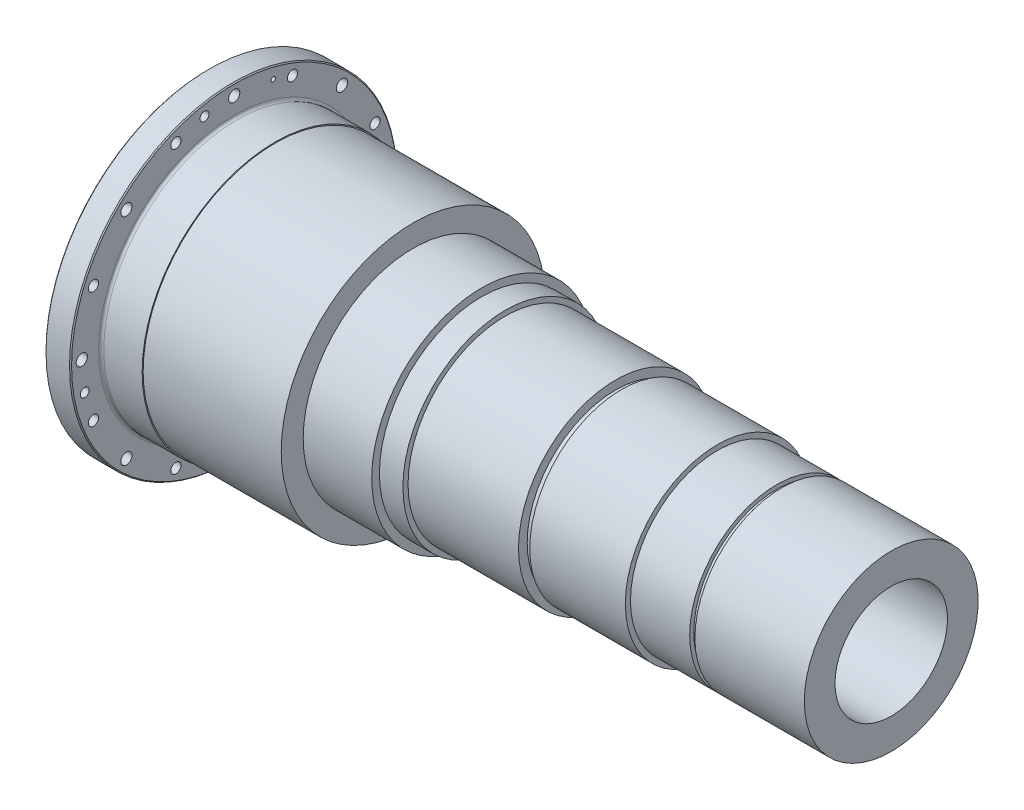
SolidWorks part; units mm, degrees
material "1.2311 (40CrMnMo7)"
ref_plane "Front Plane" through (0, 0, 0) normal (0, 0, 1) x (1, 0, 0)
ref_plane "Top Plane" through (0, 0, 0) normal (0, 1, 0) x (1, 0, 0)
ref_plane "Right Plane" through (0, 0, 0) normal (1, 0, 0) x (0, 0, -1)
sketch "Sketch1" plane through (0, 0, 0) normal (0, 0, 1) x (1, 0, 0)
  line L0 (0, 0) -> (1527.2972, 0) construction
  line L1 (0, 203) -> (0, 318)
  line L2 (2, 320) -> (48, 320)
  line L3 (50, 318) -> (50, 265)
  line L4 (55, 260) -> (130, 260)
  line L5 (130, 260) -> (130, 258)
  line L6 (130, 258) -> (400, 258)
  line L7 (400, 258) -> (400, 215)
  line L8 (400, 215) -> (534, 215)
  line L9 (534, 215) -> (534, 200)
  line L10 (534, 200) -> (580, 200)
  line L11 (580, 200) -> (580, 190)
  line L12 (580, 190) -> (796, 190)
  line L13 (796, 190) -> (796, 173)
  line L14 (796, 173) -> (808, 173)
  line L15 (808, 173) -> (808, 180)
  line L16 (808, 180) -> (995, 180)
  line L17 (995, 180) -> (995, 170)
  line L18 (995, 170) -> (1110.8, 170)
  line L19 (1110.8, 170) -> (1110.8, 162)
  line L21 (1335, 170) -> (1335, 110)
  line L22 (1335, 110) -> (874, 110)
  line L23 (874, 110) -> (864, 120)
  line L24 (864, 120) -> (413, 120)
  line L25 (413, 120) -> (413, 107.5)
  line L26 (413, 107.5) -> (353, 107.5)
  line L27 (353, 107.5) -> (353, 159)
  line L28 (353, 159) -> (340, 159)
  line L29 (340, 159) -> (340, 185)
  line L30 (340, 185) -> (283, 185)
  line L31 (283, 185) -> (283, 200)
  line L32 (278, 205) -> (175, 205)
  line L33 (170, 200) -> (170, 190)
  line L34 (170, 190) -> (110, 190)
  line L35 (110, 190) -> (110, 197)
  line L36 (107, 200) -> (3, 200)
  line L37 (1110.8, 162) -> (1121, 162)
  line L38 (1121, 162) -> (1121, 170)
  line L39 (1121, 170) -> (1335, 170)
  line L40 (3, 200) -> (0, 203)
  line L41 (0, 318) -> (2, 320)
  line L42 (48, 320) -> (50, 318)
  arc A0 (50, 265) -> (55, 260) centre (55, 265) ccw
  arc A1 (110, 197) -> (107, 200) centre (107, 197) ccw
  arc A2 (283, 200) -> (278, 205) centre (278, 200) ccw
  arc A3 (175, 205) -> (170, 200) centre (175, 200) ccw
  point P4 (0, 320)
  point P5 (50, 320)
  point P39 (0, 200)
  dimension "D38" = 5
  dimension "D39" = 3
  dimension "D43" = 5
  dimension "D1" = 320
  dimension "D2" = 1335
  dimension "D3" = 10.2
  dimension "D4" = 325
  dimension "D5" = 162
  dimension "D6" = 170
  dimension "D7" = 180
  dimension "D8" = 199
  dimension "D9" = 173
  dimension "D10" = 12
  dimension "D11" = 110
  dimension "D12" = 995
  dimension "D13" = 190
  dimension "D14" = 120
  dimension "D15" = 45
  dimension "D16" = 864
  dimension "D17" = 46
  dimension "D18" = 534
  dimension "D19" = 200
  dimension "D20" = 215
  dimension "D21" = 107.5
  dimension "D22" = 200
  dimension "D23" = 190
  dimension "D24" = 110
  dimension "D25" = 60
  dimension "D26" = 113
  dimension "D27" = 205
  dimension "D28" = 185
  dimension "D29" = 60
  dimension "D30" = 353
  dimension "D31" = 13
  dimension "D32" = 159
  dimension "D33" = 400
  dimension "D34" = 258
  dimension "D35" = 260
  dimension "D36" = 80
  dimension "D37" = 50
revolve "Revolve1" add sketch "Sketch1" angle 360 about L0
sketch "Sketch3" plane through (0, 0, 0) normal (-1, 0, 0) x (0, 0, 1)
  line L0 (0, 0) -> (114.0397, 275.3161) construction
  line L1 (0, 0) -> (0, 298) construction
  line L2 (0, 0) -> (58.1369, 292.274) construction
  line L3 (0, 0) -> (292.274, -58.1369) construction
  line L4 (0, 0) -> (-58.1369, -292.274) construction
  line L5 (0, 0) -> (-292.274, 58.1369) construction
  line L6 (0, 0) -> (298, 0) construction
  line L7 (0, 0) -> (292.274, 58.1369) construction
  circle A0 centre (0, 0) radius 298 construction
  circle A1 centre (114.0397, 275.3161) radius 10
  circle A2 centre (0, 298) radius 11
  circle A3 centre (210.7178, 210.7178) radius 11
  circle A4 centre (275.3161, 114.0397) radius 10
  circle A5 centre (298, 0) radius 11
  circle A6 centre (275.3161, -114.0397) radius 10
  circle A7 centre (210.7178, -210.7178) radius 11
  circle A8 centre (114.0397, -275.3161) radius 10
  circle A9 centre (0, -298) radius 11
  circle A10 centre (-114.0397, -275.3161) radius 10
  circle A11 centre (-210.7178, -210.7178) radius 11
  circle A12 centre (-275.3161, -114.0397) radius 10
  circle A13 centre (-298, 0) radius 11
  circle A14 centre (-275.3161, 114.0397) radius 10
  circle A15 centre (-210.7178, 210.7178) radius 11
  circle A16 centre (-114.0397, 275.3161) radius 10
  circle A17 centre (-76.5, 288.0135) radius 4.25
  point P38 (0, 0)
  point P43 (0, 0)
  dimension "D1" = 596
  dimension "D3" = 22
  dimension "D4" = 20
  dimension "D5" = 8
  dimension "D9" = 8.5
  dimension "D10" = 76.5
  dimension "D2" = 22.5
  dimension "D6" = 11.25
  dimension "D8" = 11.25
  dimension "D7" = 4
hole_wizard "M12 Tapped Hole1" positions "3DSketch2" profile "Sketch5" tap size "M12" standard "GB"
sketch3d "3DSketch2"
  point P0 (0, 58.1369, 292.274)
sketch "Sketch5" plane through (0, 58.1369, 292.274) normal (0, 1, 0) x (0, 0, 1)
  line L0 (0, 0) -> (0, 25.0644)
  line L1 (0, 25.0644) -> (5.1, 22)
  line L2 (5.1, 22) -> (5.1, 0)
  line L5 (5.1, 0) -> (0, 0)
  line L10 (0, 25.0644) -> (-5.1, 22) construction
  line L11 (0, -6.35) -> (0, 107.95) construction
  dimension "螺纹孔钻头直径" = 10.2
  dimension "螺纹孔钻头深度" = 22
  dimension "导头角度" = 118
cosmetic thread "CosmeticThread hole thread 1" parameters "D1"=18, "D2"=12
hole_wizard "M20 Tapped Hole1" positions "3DSketch3" profile "Sketch6" tap size "M20" standard "GB" end condition through all
sketch3d "3DSketch3"
  point P0 (0, 292.274, 58.1369)
  point P3 (0, 58.1369, -292.274)
  point P6 (0, -292.274, -58.1369)
  point P9 (0, -58.1369, 292.274)
sketch "Sketch6" plane through (0, 292.274, 58.1369) normal (0, 1, 0) x (0, 0, 1)
  line L0 (0, 0) -> (0, 1335)
  line L1 (0, 1335) -> (8.75, 1335)
  line L2 (8.75, 1335) -> (8.75, 0)
  line L5 (8.75, 0) -> (0, 0)
  line L11 (0, -6.35) -> (0, 107.95) construction
  dimension "通孔螺纹孔钻头直径" = 17.5
  dimension "通孔螺纹孔钻头深度" = 1335
cosmetic thread "CosmeticThread hole thread 2" parameters "D2"=20
cosmetic thread "CosmeticThread hole thread 3" parameters "D2"=20
cosmetic thread "CosmeticThread hole thread 4" parameters "D2"=20
cosmetic thread "CosmeticThread hole thread 5" parameters "D2"=20
extrude "Cut-Extrude2" cut sketch "Sketch3" against normal through all
sketch "Sketch7" plane through (0, 0, 0) normal (-1, 0, 0) x (0, 0, 1)
  circle A0 centre (-76.5, 288.0135) radius 11.05
  dimension "D1" = 22.1
extrude "Cut-Extrude3" cut sketch "Sketch7" against normal blind 2.75
sketch "Sketch8" plane through (0, 0, 0) normal (1, 0, 0) x (0, 0, -1)
  line L0 (0, 0) -> (0, 318) construction
  circle A0 centre (0, 0) radius 318 construction
